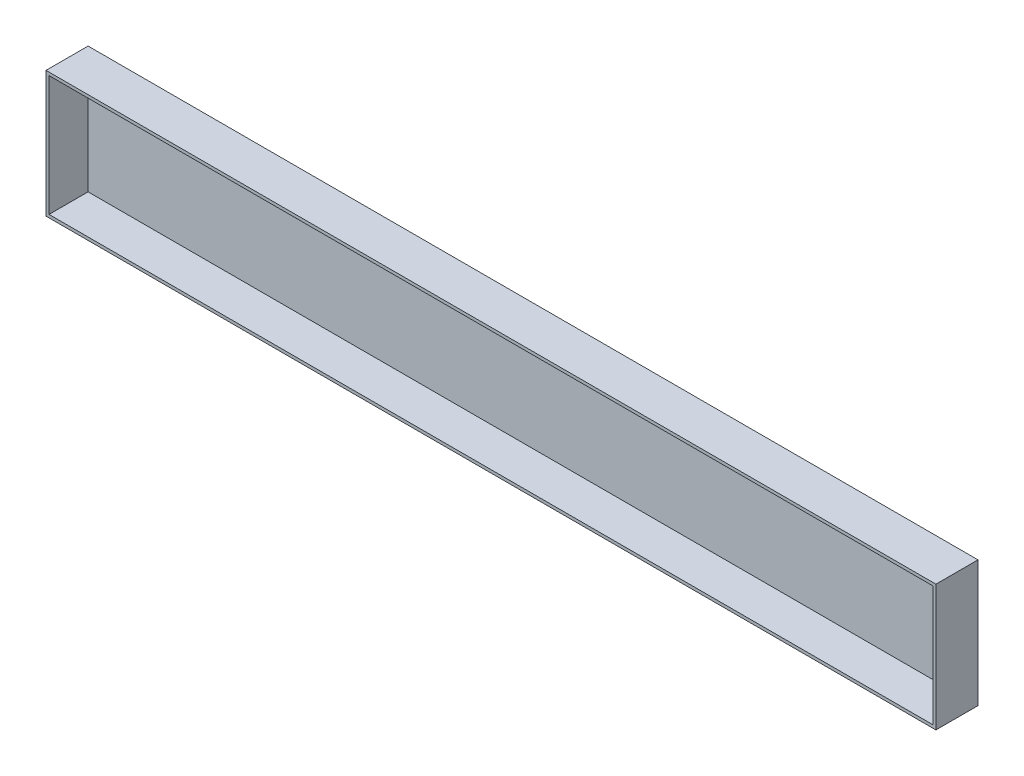
SolidWorks part; units mm, degrees
material "瓦楞纸板盒"
ref_plane "前视基准面" through (0, 0, 0) normal (0, 0, 1) x (1, 0, 0)
ref_plane "上视基准面" through (0, 0, 0) normal (0, 1, 0) x (1, 0, 0)
ref_plane "右视基准面" through (0, 0, 0) normal (1, 0, 0) x (0, 0, -1)
other "Configuration Table"
sketch "草图1" plane through (0, 0, 0) normal (0, 0, 1) x (1, 0, 0)
  line L1 (-735, -100) -> (735, -100)
  line L2 (-735, -100) -> (-735, 100)
  line L3 (-735, 100) -> (735, 100)
  line L4 (735, -100) -> (735, 100)
  line L5 (-735, -100) -> (735, 100) construction
  line L6 (-735, 100) -> (735, -100) construction
  point P0 (0, 0)
  dimension "D1" = 1470
  dimension "D2" = 200
extrude "拉伸-薄壁1" add sketch "草图1" along normal blind 70 thin
sketch "草图2" plane through (735, 0, 0) normal (-1, 0, 0) x (0, 0, 1)
  line L0 (70, -105) -> (0, -105) construction
  line L1 (0, 105) -> (5, 105)
  line L2 (0, 105) -> (0, -105)
  line L3 (0, -105) -> (5, -105)
  line L4 (5, 105) -> (5, -105)
  dimension "D1" = 5
extrude "凸台-拉伸1" add sketch "草图2" along normal up to surface (1470 mm away) up to face at (-735, 0, 35)
